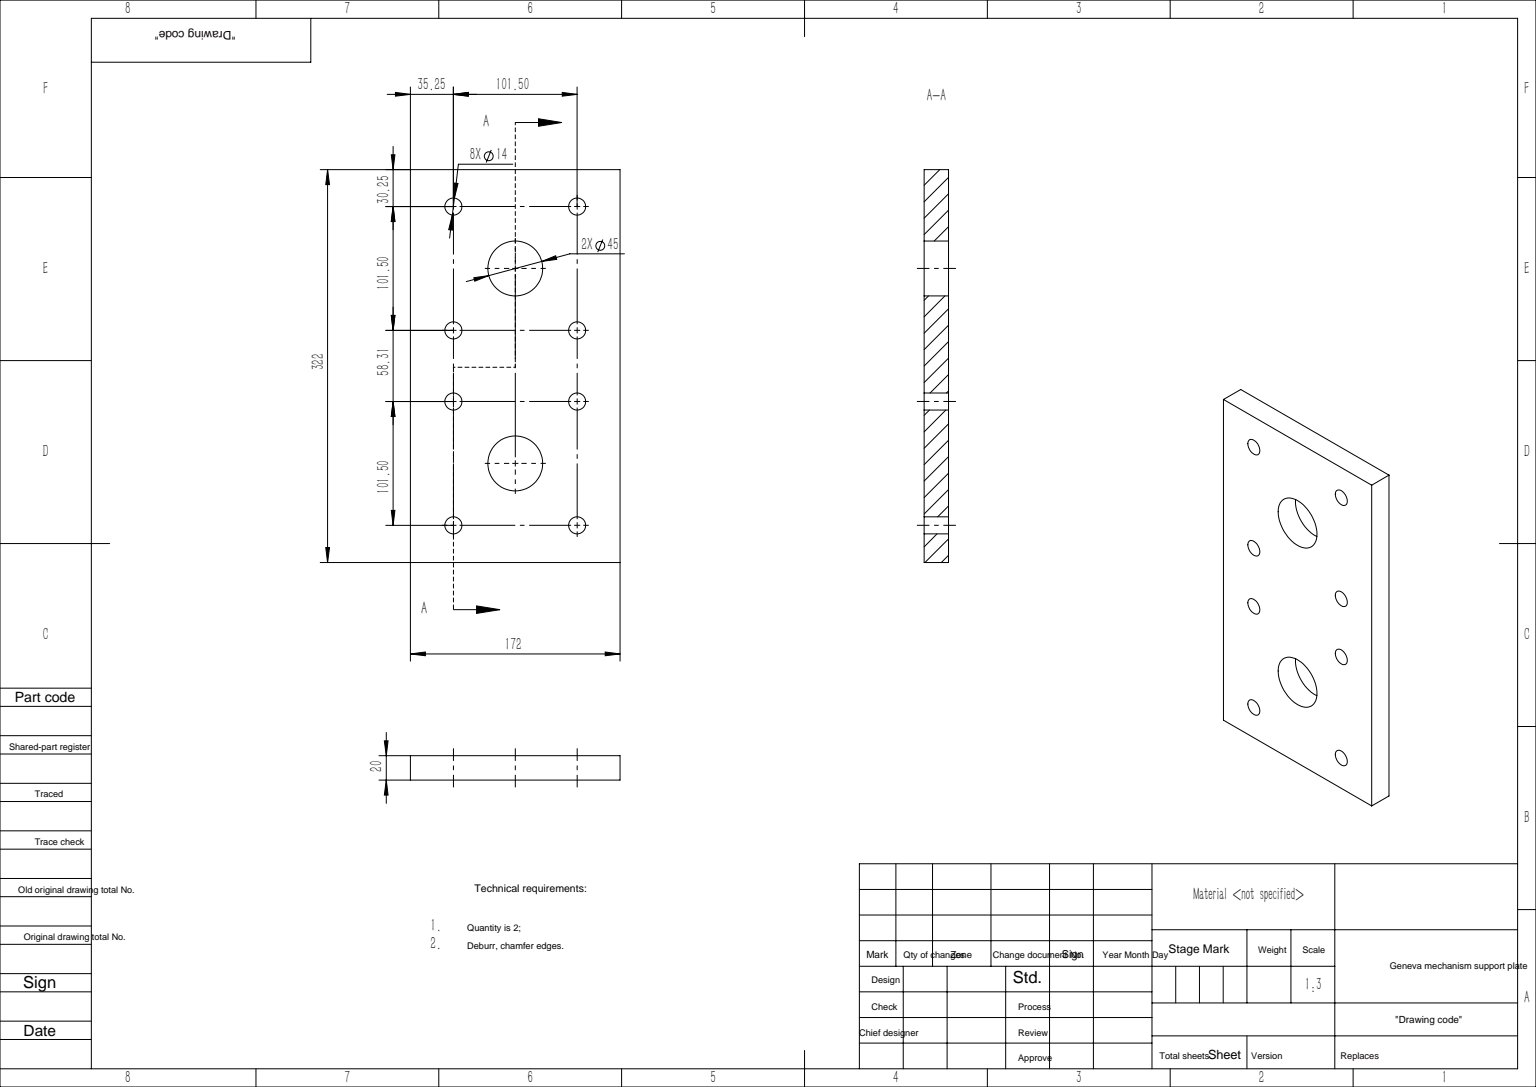
SolidWorks part; units mm, degrees
ref_plane "前视基准面" through (0, 0, 0) normal (0, 0, 1) x (1, 0, 0)
ref_plane "上视基准面" through (0, 0, 0) normal (0, 1, 0) x (1, 0, 0)
ref_plane "右视基准面" through (0, 0, 0) normal (1, 0, 0) x (0, 0, -1)
sketch "草图1" plane through (0, 0, 0) normal (0, 0, 1) x (1, 0, 0)
  line L0 (-235.4223, 0) -> (364.5777, 0) construction
  line L1 (-86, 161) -> (86, 161)
  line L2 (-86, 161) -> (-86, -161)
  line L3 (-86, -161) -> (86, -161)
  line L4 (86, 161) -> (86, -161)
  line L5 (0, 264.8501) -> (0, -335.1499) construction
  dimension "D1" = 322
  dimension "D2" = 172
  dimension "D3" = 600
  dimension "D4" = 600
extrude "凸台-拉伸1" add sketch "草图1" along normal blind 20
sketch "草图3" plane through (0, 0, 0) normal (0, 0, -1) x (-1, 0, 0)
  circle A0 centre (0, 80) radius 22.5
  circle A1 centre (-50.75, 130.75) radius 7
  circle A2 centre (50.75, 130.75) radius 7
  circle A3 centre (-50.75, 29.25) radius 7
  circle A4 centre (50.75, 29.25) radius 7
  circle A5 centre (0, -79.81) radius 22.5
  circle A6 centre (-50.75, -29.06) radius 7
  circle A7 centre (50.75, -29.06) radius 7
  circle A8 centre (50.75, -130.56) radius 7
  circle A9 centre (-50.75, -130.56) radius 7
  dimension "D1" = 45
  dimension "D2" = 14
extrude "切除-拉伸1" cut sketch "草图3" against normal through all
